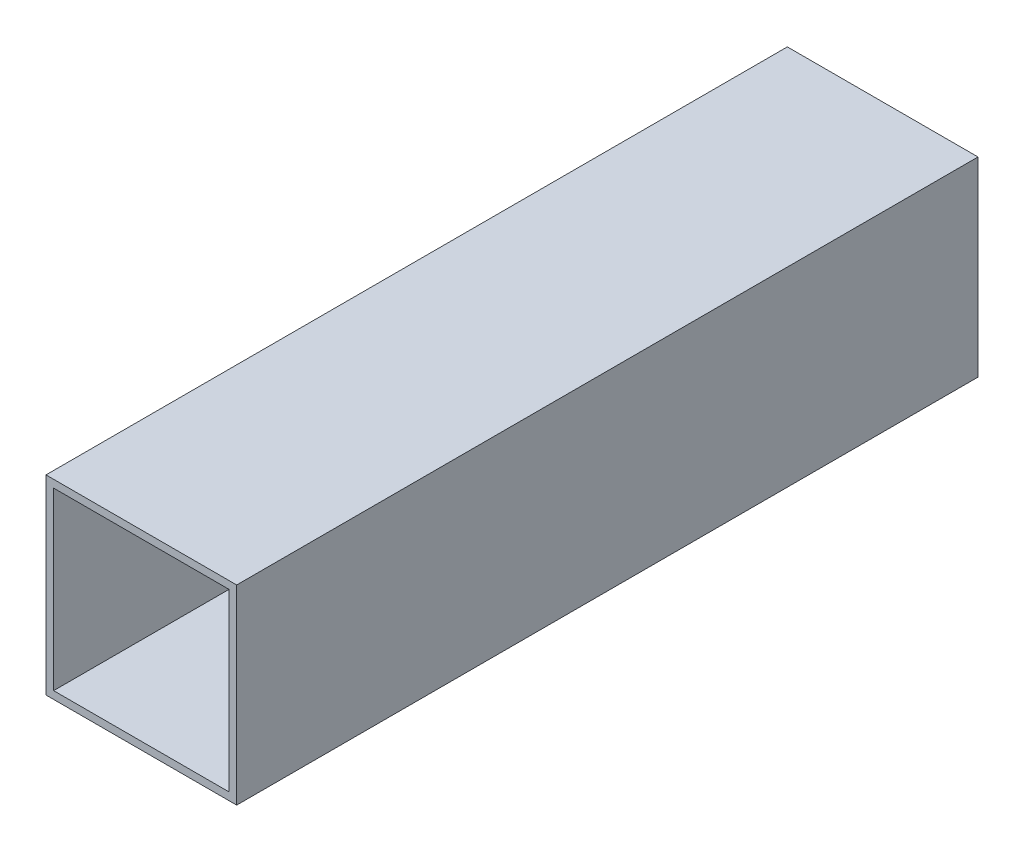
from build123d import *

# Parameters (mm, degrees)
SKETCH1_W           = 50
SKETCH1_H           = 50
SKETCH1_W_2         = 46
SKETCH1_H_2         = 46
BOSS_EXTRUDE1_DEPTH = 194.4


with BuildPart() as part:
    # Sketch1 → Boss-Extrude1 (new body)
    with BuildSketch(Plane.XY):
        Rectangle(SKETCH1_W, SKETCH1_H)
        Rectangle(SKETCH1_W_2, SKETCH1_H_2, mode=Mode.SUBTRACT)
    extrude(amount=BOSS_EXTRUDE1_DEPTH)


solid = part.part
